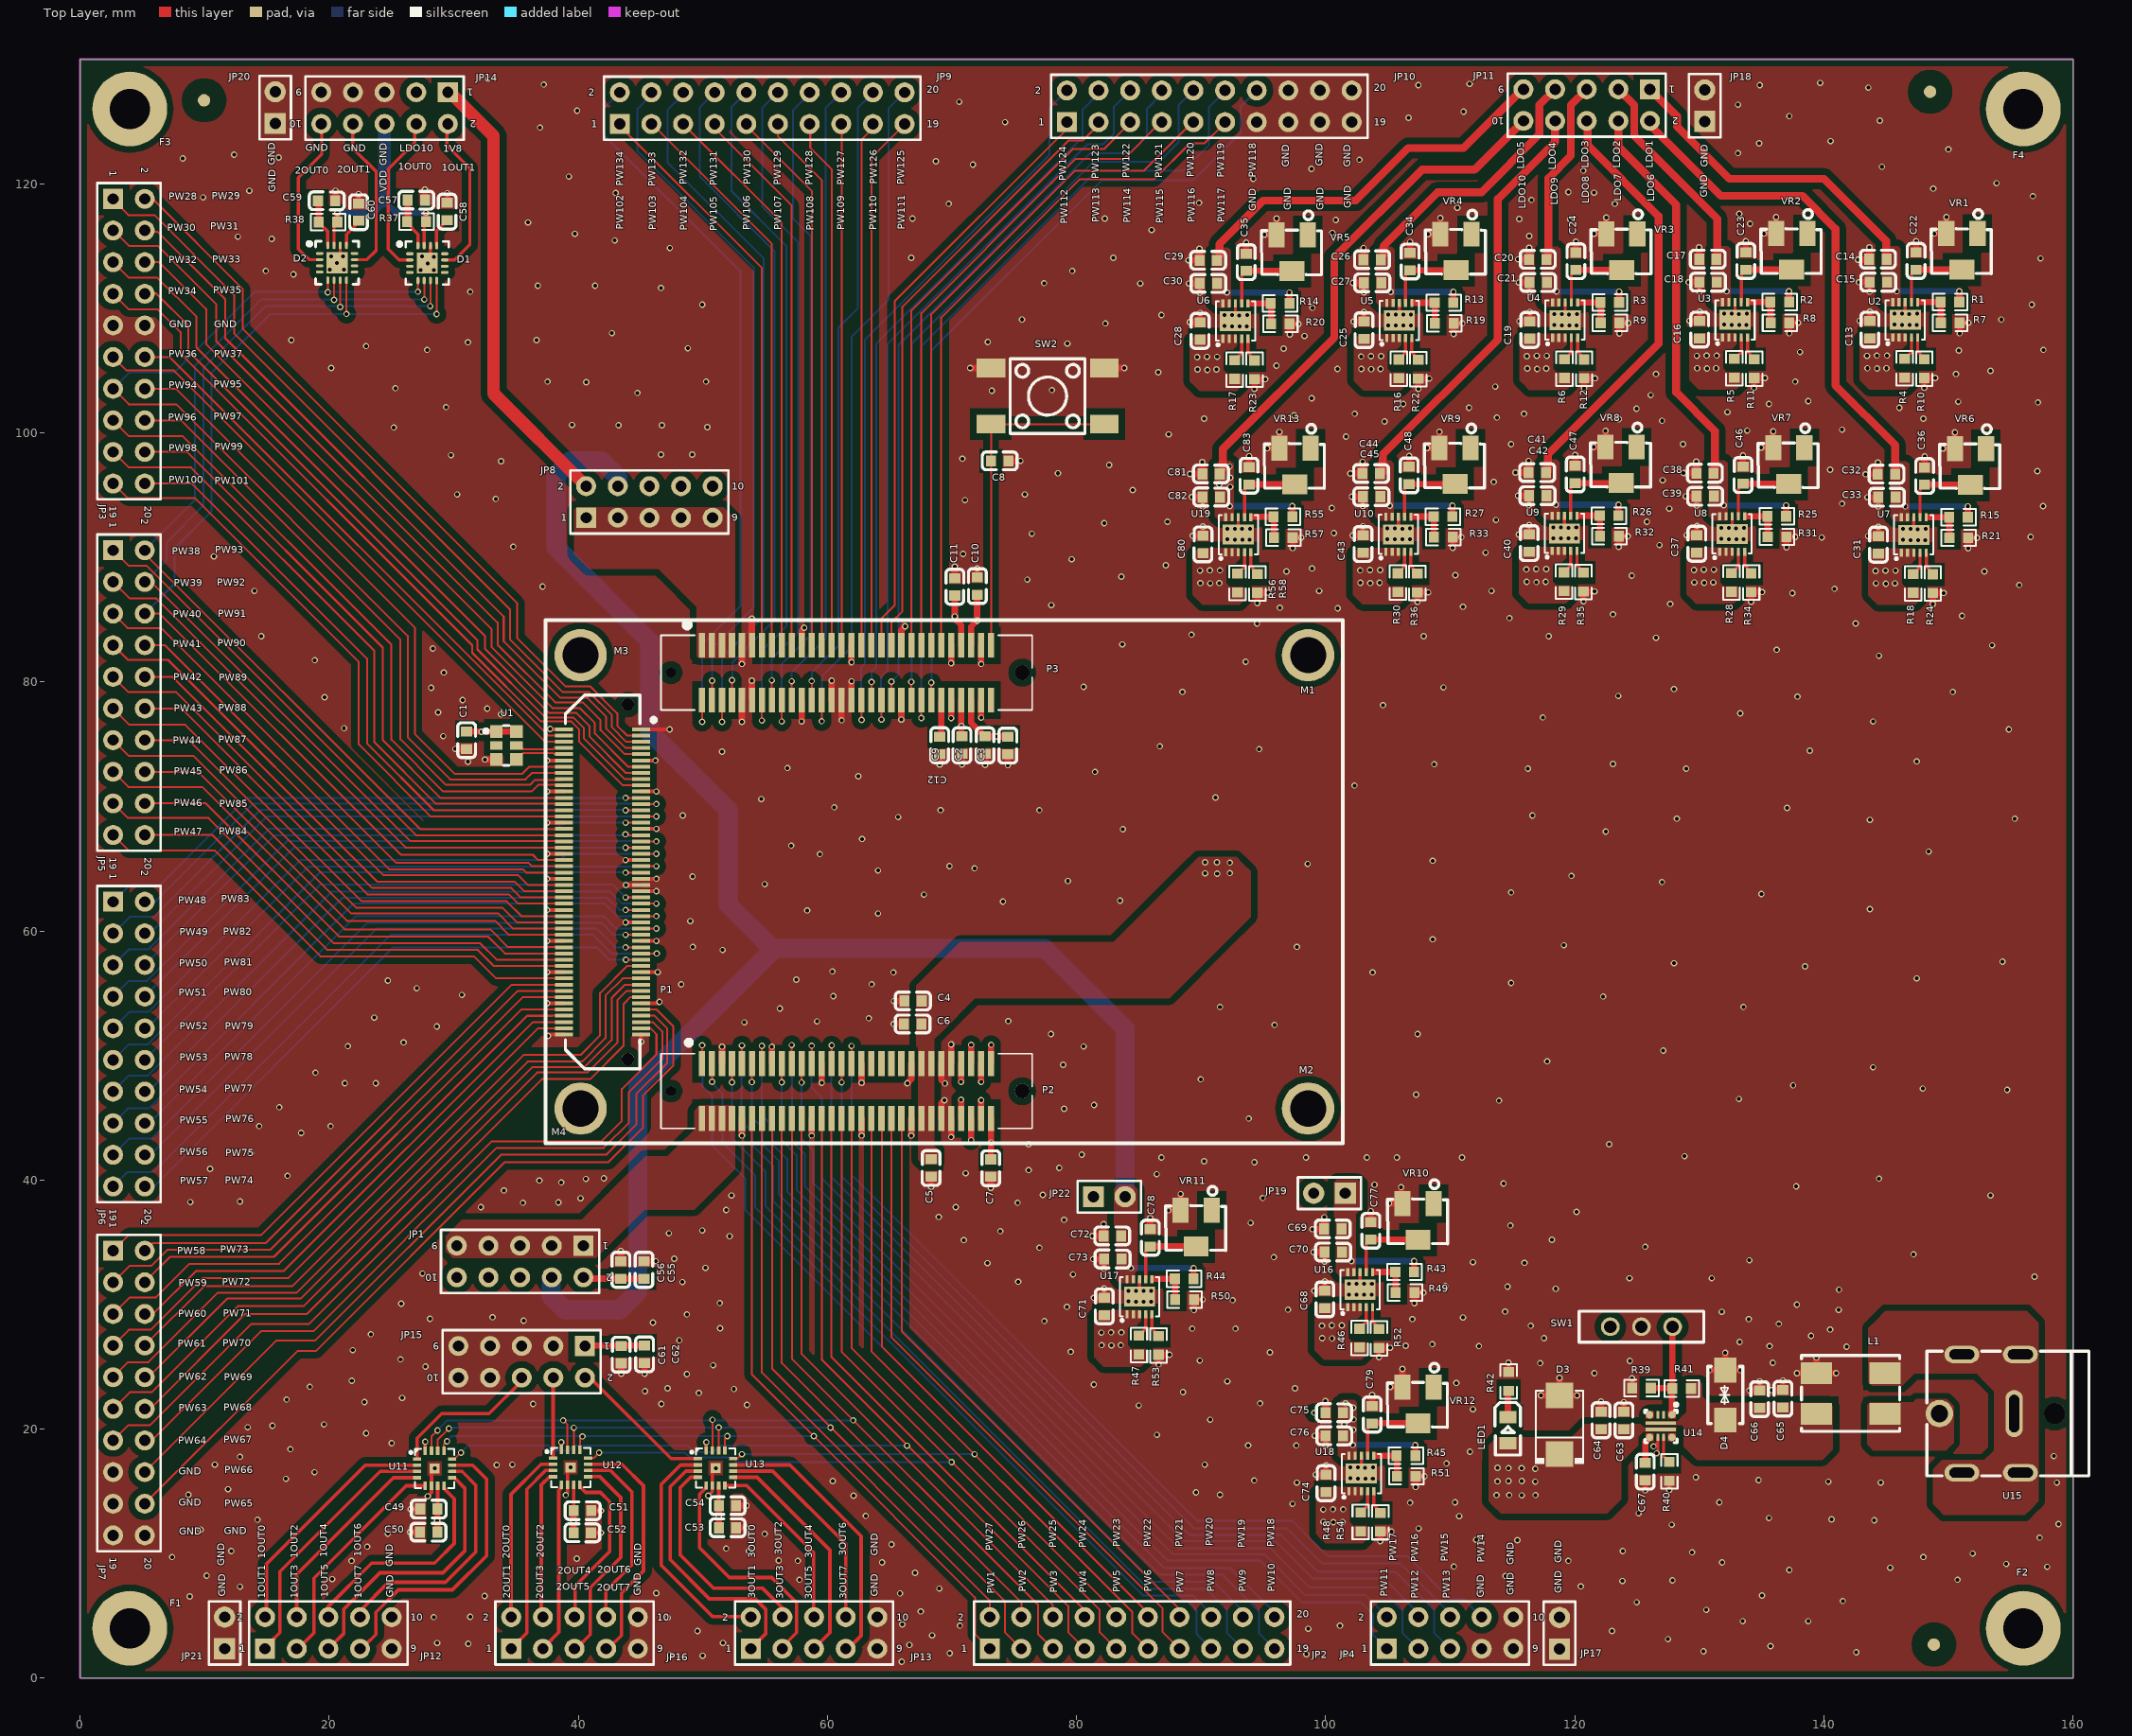
[diagram p0: Top Layer view]
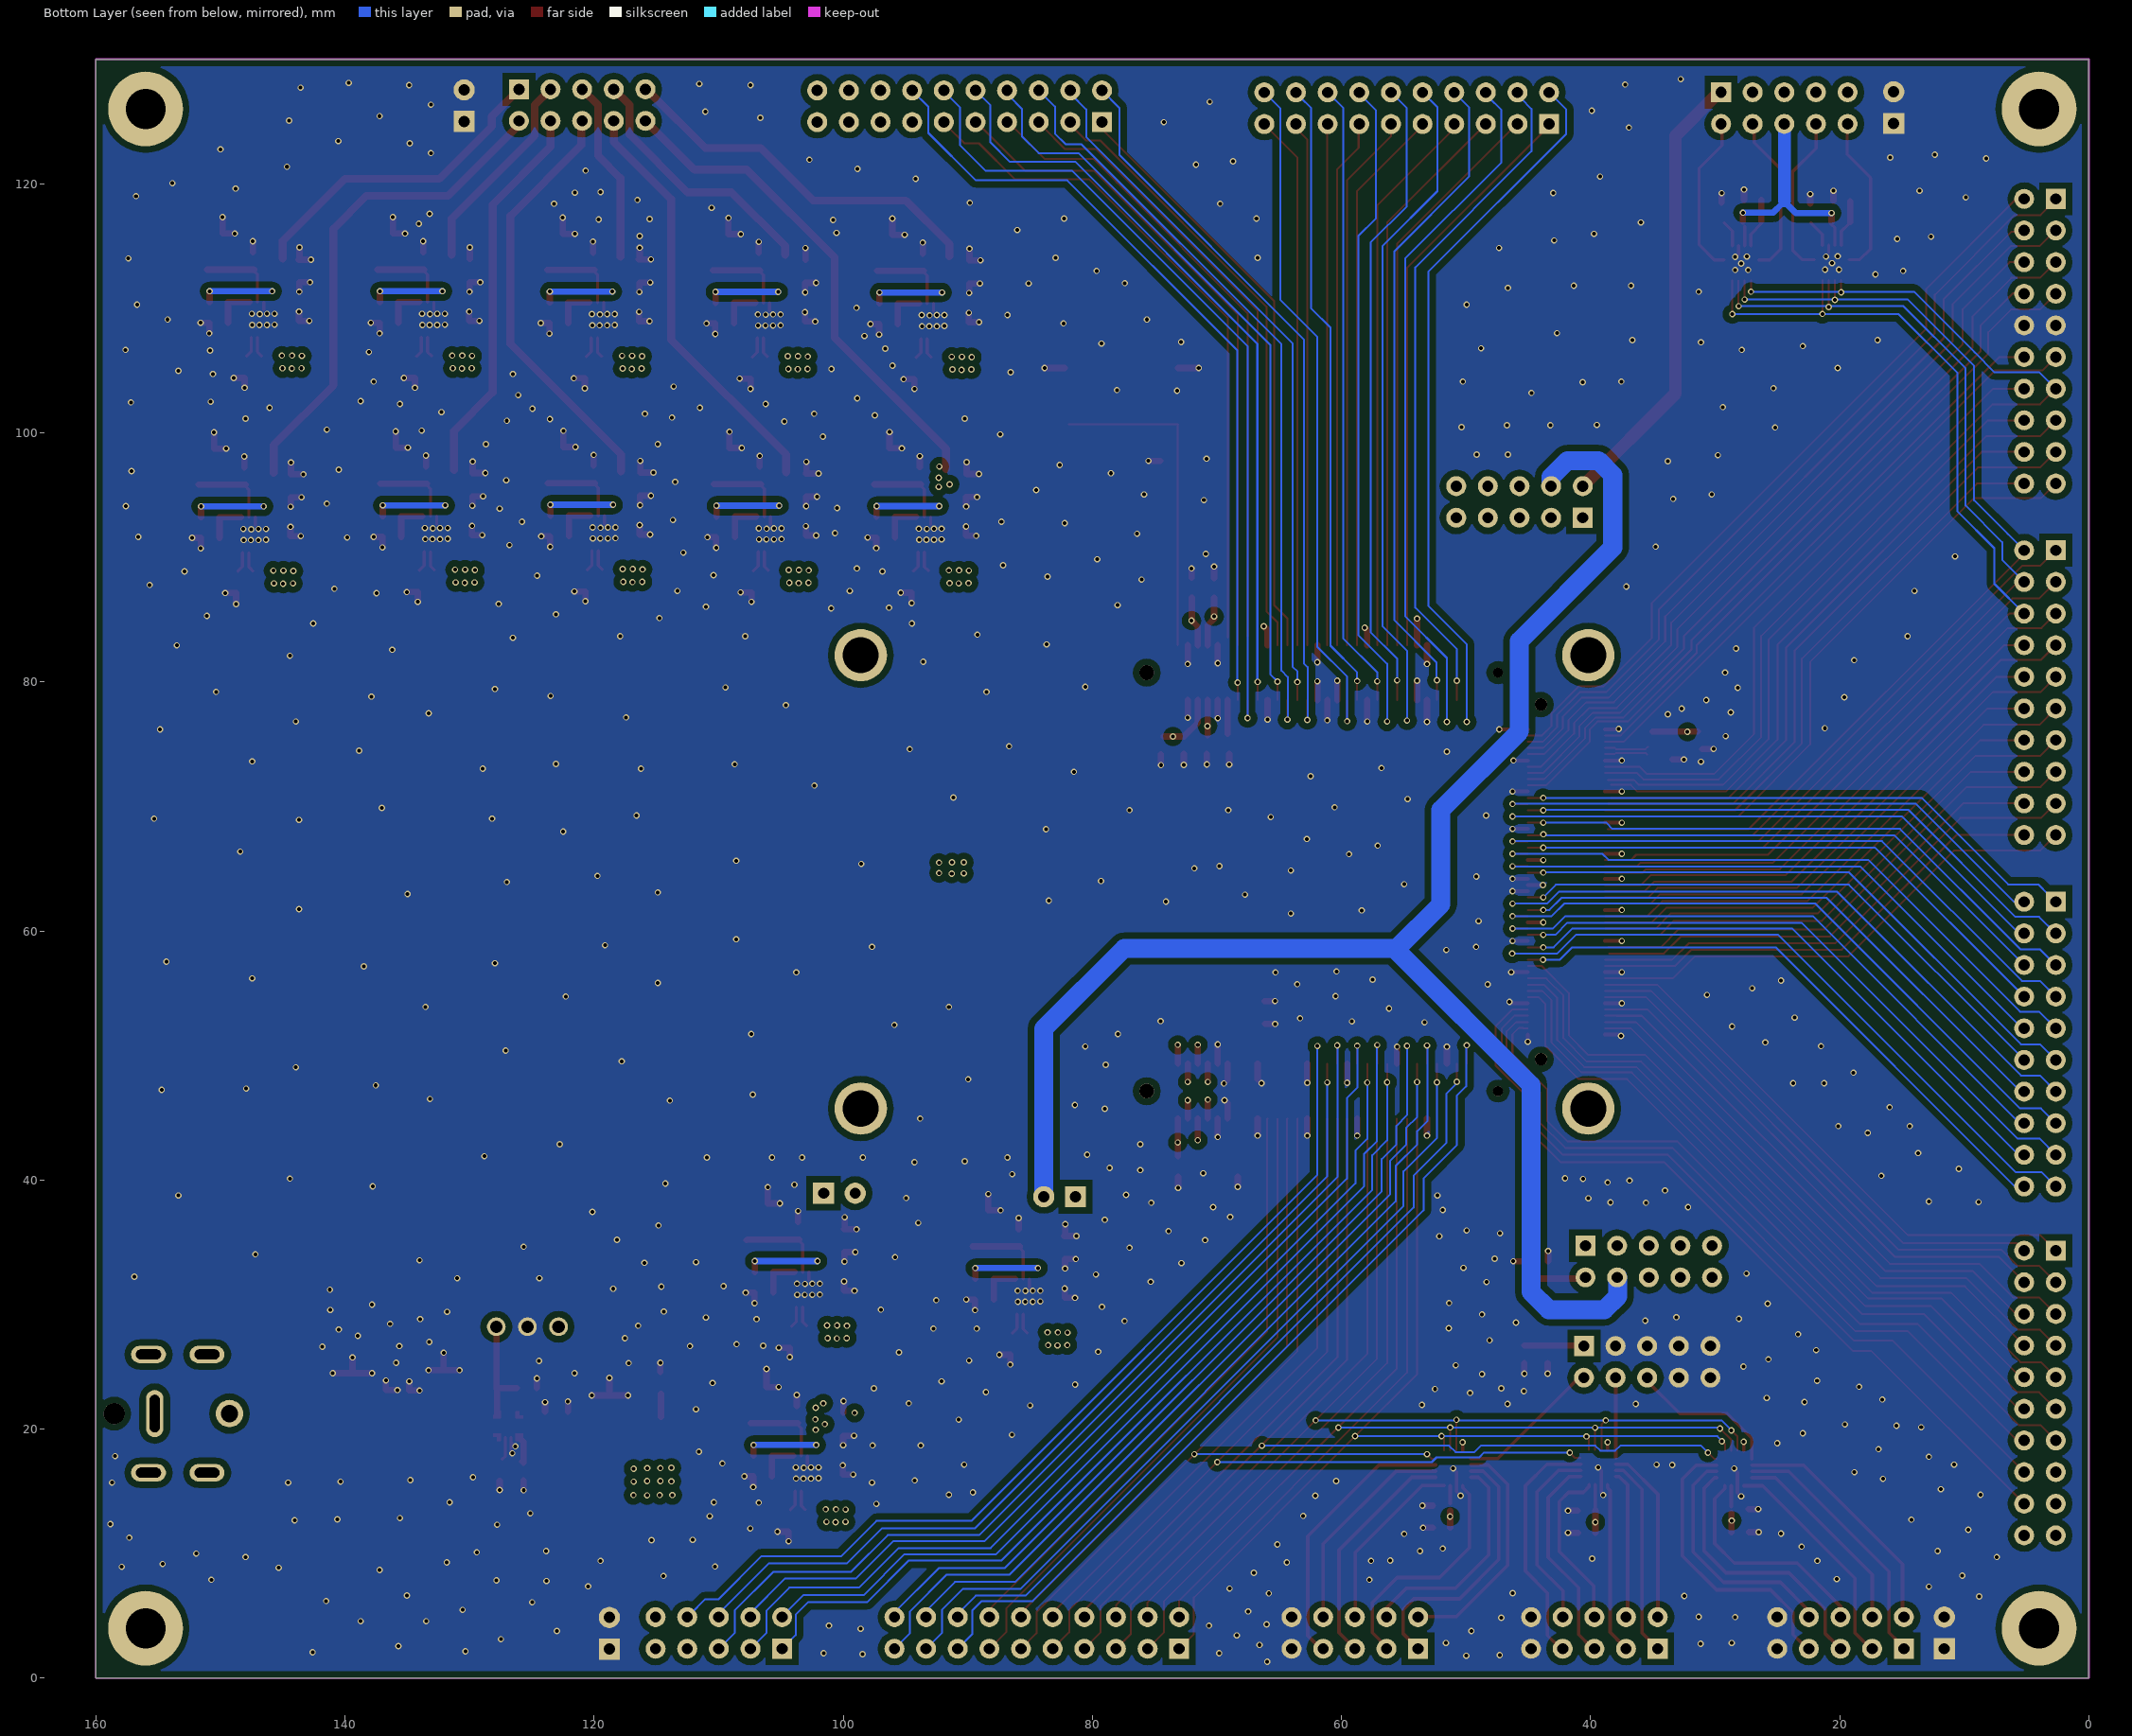
[diagram p1: Bottom Layer view, seen from below]
# Altium PCB MISC82195.PcbDoc (part 1 of 8)
Units mm, origin at the board's own origin, x right, y up, seen from the top; angles counter-clockwise.
Board outline 160 x 130 mm, 4 copper layers (Top Layer, GND, POWER, Bottom Layer); 214 components, 251 nets, 1068 pads, 1218 vias.

## Layer stack, top to bottom (the 12.6 mil dielectric is the usual default, probably not edited)
Top Layer: signal copper 0.0356
Dielectric: core 0.32, FR-4, Dk 4.8
GND: plane copper 0.0356, net GND
Dielectric: prepreg 0.32, FR-4, Dk 4.8
POWER: plane copper 0.0356, net LDO_10
Dielectric: core 0.32, FR-4, Dk 4.8
Bottom Layer: signal copper 0.0356

## Board outline
0,0 160,0 160,130 0,130

## Design rules (kind name [scope] priority, off if disabled: settings)
Clearance Clearance_2 [HASPAD('FREE-MARK')] p1: gap=1.27
Clearance Clearance_1 [INPOLYGON] p2: gap=0.152
Clearance [All] p3: gap=0.152
DiffPairsRouting [All] p1: maxlimit=0.152 minlimit=0.152 mostfreqgap=0.152 maxuncoupledlength=12.7
HoleSize [All] p1: absolutevalues=TRUE maxlimit=12.7 minlimit=0.025 maxpercent=80.000 minpercent=20.000
HoleToHoleClearance [All] p1: gap=0 allowstackedmicrovias=TRUE
MinimumSolderMaskSliver [All] p1: minsoldermaskwidth=0
PlaneClearance [All] p1: clearance=0.152
PlaneConnect [All] p1: planeconnectstyle=Direct reliefexpansion=0.508 reliefentries=4 reliefconductorwidth=0.254 reliefairgap=0.254
PolygonConnect [All] p1: connectstyle=Direct reliefconductorwidth=0.254 reliefentries=4 polygonreliefangle="90 Angle"
RoutingVias [All] p1: holewidth=0.305 width=0.508 viastyle="Through Hole" minholewidth=0.305 minwidth=0.508 maxholewidth=0.305 maxwidth=0.508
SilkToSilkClearance [All] p1: silktosilkclearance=0
SilkscreenOverComponentPads [All] p1: minsilkscreentomaskgap=0
SolderMaskExpansion [All] p1: expansion=0.102
Width [All] p1: maxlimit=2.032 minlimit=0.152 preferedwidth=0.152 minimp=50.000000 maximp=50.000000 favimp=50.000000
20 further rules are at their usual default settings.

## Classes and differential pairs
component class AnalogSignal: C13 C14 C15 C16 C17 C18 C19 C20 C21 C22 C23 C24 C25 C26 C27 C28 C29 C30 C31 C32 C33 C34 C35 C36 C37 C38 C39 C40 C41 C42 C43 C44 C45 C46 C47 C48 C49 C50 C51 C52 C53 C54 C55 C56 C57 C58 C59 C60 C61 C62 C80 C81 C82 C83 C? D1 D2 JP11 JP12 JP13 JP14 JP15 JP16 R1 R2 R3 R4 R5 R6 R7 R8 R9 R10 R11 R12 R13 R14 R15 R16 R17 R18 R19 R20 R21 R22 R23 R24 R25 R26 R27 R28 R29 R30 R31 R32 R33 R34 R35 R36 R37 R38 R55 R56 R57 R58 R? U2 U3 U4 U5 U6 U7 U8 U9 U10 U11 U12 U13 U19 VR1 VR2 VR3 VR4 VR5 VR6 VR7 VR8 VR9 VR13
component class FPGA: C1 C2 C3 C4 C5 C6 C7 C8 C9 C10 C11 C12 F1 F2 F3 F4 JP1 JP2 JP3 JP4 JP5 JP6 JP7 JP8 JP9 JP10 P1 P2 P3 SW2 U1
component class Power: C63 C64 C65 C66 C67 C68 C69 C70 C71 C72 C73 C74 C75 C76 C77 C78 C79 D3 D4 JP17 JP18 JP19 JP20 JP21 JP22 L1 LED1 M1 M2 M3 M4 R39 R40 R41 R42 R43 R44 R45 R46 R47 R48 R49 R50 R51 R52 R53 R54 SW1 U14 U15 U16 U17 U18 VR10 VR11 VR12

## Components (designator, comment, footprint, x,y, rotation, side; value= is the part's Value field where it differs from the comment)
C1 "X7R  100nF/16V" C0603 31.039,75.311 r270 top
C2 "100nF/50V" C0603 72.66,74.915 r90 top
C3 "22uF/10V" C0603 74.489,74.889 r90 top
C4 "100nF/50V" C0603 66.868,54.372 r0 top
C5 "22uF/10V" C0603 68.326,40.97 r90 top
C6 "100nF/50V" C0603 66.853,52.527 r0 top
C7 "100nF/50V" C0603 73.117,40.955 r90 top
C8 "100nF" C0603 73.838,97.739 r0 top
C9 "100nF/50V" C0603 70.806,74.915 r90 top
C10 "100nF/50V" C0603 72.034,87.681 r270 top
C11 "22uF/10V" C0603 70.231,87.63 r270 top
C12 "100nF/50V" C0603 69.012,74.905 r270 top
C13 "10uF" C0603 143.688,108.28 r270 top
C14 "10uF" C0603 144.34,113.944 r0 top
C15 "10uF" C0603 144.366,112.09 r0 top
C16 "10uF" C0603 130.023,108.28 r270 top
C17 "10uF" C0603 130.675,113.944 r0 top
C18 "10uF" C0603 130.701,112.09 r0 top
C19 "10uF" C0603 116.383,108.255 r270 top
C20 "10uF" C0603 117.035,113.919 r0 top
C21 "10uF" C0603 117.061,112.065 r0 top
C22 "4.7uF" C0603 147.388,113.792 r270 top
C23 "4.7uF" C0603 133.723,113.792 r270 top
C24 "4.7uF" C0603 120.083,113.767 r270 top
C25 "10uF" C0603 103.073,108.229 r270 top
C26 "10uF" C0603 103.726,113.894 r0 top
C27 "10uF" C0603 103.751,112.039 r0 top
C28 "10uF" C0603 89.916,108.179 r270 top
C29 "10uF" C0603 90.569,113.843 r0 top
C30 "10uF" C0603 90.594,111.989 r0 top
C31 "10uF" C0603 144.374,91.008 r270 top
C32 "10uF" C0603 145.026,96.672 r0 top
C33 "10uF" C0603 145.052,94.818 r0 top
C34 "4.7uF" C0603 106.774,113.741 r270 top
C35 "4.7uF" C0603 93.617,113.69 r270 top
C36 "4.7uF" C0603 148.074,96.52 r270 top
C37 "10uF" C0603 129.794,91.084 r270 top
C38 "10uF" C0603 130.447,96.749 r0 top
C39 "10uF" C0603 130.472,94.894 r0 top
C40 "10uF" C0603 116.332,91.135 r270 top
C41 "10uF" C0603 116.985,96.799 r0 top
C42 "10uF" C0603 117.01,94.945 r0 top
C43 "10uF" C0603 102.997,91.059 r270 top
C44 "10uF" C0603 103.65,96.723 r0 top
C45 "10uF" C0603 103.675,94.869 r0 top
C46 "4.7uF" C0603 133.495,96.596 r270 top
C47 "4.7uF" C0603 120.033,96.647 r270 top
C48 "4.7uF" C0603 106.698,96.571 r270 top
C49 "10uF" C0603 28.007,13.574 r0 top
C50 "100nF" C0603 27.982,11.72 r0 top
C51 "10uF" C0603 40.344,13.452 r180 top
C52 "100nF" C0603 40.319,11.674 r180 top
C53 "10uF" C0603 51.978,12.08 r180 top
C54 "100nF" C0603 51.978,13.858 r180 top
C55 "0.1uF/16V" C0603 45.272,32.781 r270 top
C56 "0.1uF/16V" C0603 43.418,32.781 r270 top
C57 "100nF" C0603 26.991,118.679 r180 top
C58 "1.5uF" C0603 29.48,117.765 r90 top
C59 "100nF" C0603 19.803,118.628 r180 top
C60 "1.5uF" C0603 22.368,117.714 r90 top
C61 "10uF" C0603 43.443,25.985 r90 top
C62 "10nF" C0603 45.323,26.011 r90 top
C63 "22uF/10V" C0603 123.936,20.691 r270 top
C64 "22uF/10V" C0603 122.098,20.701 r270 top
C65 "X7R 100nF/25V" C0603 136.703,22.428 r270 top
C66 "X7R 100nF/25V" C0603 134.832,22.393 r270 top
C67 "X7R" C0603 125.654,16.586 r90 top
C68 "10uF" C0603 99.924,30.404 r270 top
C69 "10uF" C0603 100.576,36.068 r0 top
C70 "10uF" C0603 100.602,34.214 r0 top
C71 "10uF" C0603 82.22,29.845 r270 top
C72 "10uF" C0603 82.872,35.509 r0 top
C73 "10uF" C0603 82.898,33.655 r0 top
C74 "10uF" C0603 100.025,15.646 r270 top
C75 "10uF" C0603 100.678,21.311 r0 top
C76 "10uF" C0603 100.703,19.456 r0 top
C77 "4.7uF" C0603 103.624,35.916 r270 top
C78 "4.7uF" C0603 85.92,35.357 r270 top
C79 "4.7uF" C0603 103.726,21.158 r270 top
C80 "10uF" C0603 90.145,91.034 r270 top
C81 "10uF" C0603 90.797,96.698 r0 top
C82 "10uF" C0603 90.823,94.844 r0 top
C83 "4.7uF" C0603 93.845,96.545 r270 top
D1 "DAC53202" WQFN-16(3x3) 27.88,113.624 r0 top
D2 "DAC53202" WQFN-16(3x3) 20.641,113.65 r0 top
D3 "#NAME?" SMB_L4.6-W3.6-LS5.3-RD 118.77,20.345 r90 top
D4 "#NAME?" SMA_L4.2-W2.7-LS5.0-BI 132.08,22.733 r270 top
F1 "M3" M3 4,4 r0 top
F2 "M3" M3 156,4 r0 top
F3 "M3" M3 4,126 r0 top
F4 "M3" M3 156,126 r0 top
JP1 "Header 5X2" HDR2.54-LI-2x5P 35.331,33.452 r180 top
JP2 "Header 2X10" HDR2.54-LI-2x10P 84.455,3.632 r0 top
JP3 "Header 2X10" HDR2.54-LI-2x10P 3.928,107.351 r270 top
JP4 "Header 5X2" HDR2.54-LI-2x5P 109.982,3.632 r0 top
JP5 "Header 2X10" HDR2.54-LI-2x10P 3.928,79.131 r270 top
JP6 "Header 2X10" HDR2.54-LI-2x10P 3.928,50.912 r270 top
JP7 "Header 2X10" HDR2.54-LI-2x10P 3.928,22.896 r270 top
JP8 "Header 5X2" HDR2.54-LI-2x5P 45.711,94.447 r0 top
JP9 "Header 2X10" HDR2.54-LI-2x10P 54.762,126.06 r0 top
JP10 "Header 2X10" HDR2.54-LI-2x10P 90.653,126.213 r0 top
JP11 "Header 5X2" HDR2.54-LI-2x5P 120.955,126.314 r180 top
JP12 "Header 5X2" HDR2.54-LI-2x5P 19.939,3.632 r0 top
JP13 "Header 5X2" HDR2.54-LI-2x5P 58.928,3.632 r0 top
JP14 "Header 5X2" HDR2.54-LI-2x5P 24.451,126.07 r180 top
JP15 "Header 5X2" HDR2.54-LI-2x5P 35.458,25.4 r180 top
JP16 "Header 5X2" HDR2.54-LI-2x5P 39.7,3.632 r0 top
JP17 "HDR-1X2" HDR2.54-LI-2P 118.77,3.607 r90 top
JP18 "HDR-1X2" HDR2.54-LI-2P 130.429,126.263 r90 top
JP19 "HDR-1X2" HDR2.54-LI-2P 100.305,38.938 r180 top
JP20 "HDR-1X2" HDR2.54-LI-2P 15.672,126.111 r90 top
JP21 "HDR-1X2" HDR2.54-LI-2P 11.608,3.632 r90 top
JP22 "HDR-1X2" HDR2.54-LI-2P 82.626,38.659 r0 top
L1 "#NAME?" FILTER-SMD_4P-L7.0-W6.0-TL_SMCM7060 142.138,22.86 r180 top
LED1 "#NAME?" LED0805-R-RD 114.63,19.914 r270 top
M1 "M2-4-L5-1.6" M2.9 83.167,80.738 r0 top
M2 "M2-4-L5-1.6" M2.9 83.167,44.338 r0 top
M3 "M2-4-L5-1.6" M2.9 24.767,80.738 r0 top
M4 "M2-4-L5-1.6" M2.9 24.767,44.338 r0 top
P1 "XMS6302-B" XMS6302-B 41.952,63.938 r270 top locked
P2 "XMS6302-A" XMS6302-A 61.537,47.138 r0 top locked
P3 "XMS6302-C" XMS6302-C 61.537,80.739 r0 top locked
R1 "453k" R0603 150.106,110.49 r0 top
R2 "453k" R0603 136.441,110.49 r0 top
R3 "453k" R0603 122.801,110.465 r0 top
R4 "200k" R0603 146.474,105.181 r270 top
R5 "200k" R0603 132.809,105.181 r270 top
R6 "200k" R0603 119.169,105.156 r270 top
R7 "50k" R0603 150.132,108.839 r180 top
R8 "50k" R0603 136.466,108.839 r180 top
R9 "50k" R0603 122.827,108.814 r180 top
R10 "249R" R0603 148.049,105.156 r90 top
R11 "249R" R0603 134.384,105.156 r90 top
R12 "249R" R0603 120.744,105.131 r90 top
R13 "453k" R0603 109.492,110.439 r0 top
R14 "453k" R0603 96.334,110.388 r0 top
R15 "453k" R0603 150.792,93.218 r0 top
R16 "200k" R0603 105.859,105.131 r270 top
R17 "200k" R0603 92.702,105.08 r270 top
R18 "200k" R0603 147.16,87.909 r270 top
R19 "50k" R0603 109.517,108.788 r180 top
R20 "50k" R0603 96.36,108.737 r180 top
R21 "50k" R0603 150.817,91.567 r180 top
R22 "249R" R0603 107.434,105.105 r90 top
R23 "249R" R0603 94.277,105.054 r90 top
R24 "249R" R0603 148.735,87.884 r90 top
R25 "453k" R0603 136.212,93.294 r0 top
R26 "453k" R0603 122.75,93.345 r0 top
R27 "453k" R0603 109.415,93.269 r0 top
R28 "200k" R0603 132.58,87.986 r270 top
R29 "200k" R0603 119.118,88.036 r270 top
R30 "200k" R0603 105.783,87.96 r270 top
R31 "50k" R0603 136.238,91.643 r180 top
R32 "50k" R0603 122.776,91.694 r180 top
R33 "50k" R0603 109.441,91.618 r180 top
R34 "249R" R0603 134.155,87.96 r90 top
R35 "249R" R0603 120.693,88.011 r90 top
R36 "249R" R0603 107.358,87.935 r90 top
R37 "10K" R0603 27.016,116.952 r0 top
R38 "10K" R0603 19.904,116.926 r0 top
R39 "357K" R0603 125.349,23.292 r180 top
R40 "681Ω" R0603 127.584,16.612 r270 top
R41 "1M" R0603 128.575,23.266 r180 top
R42 "10K" R0603 114.681,23.825 r270 top
R43 "453k" R0603 106.342,32.614 r0 top
R44 "453k" R0603 88.638,32.055 r0 top
R45 "453k" R0603 106.444,17.856 r0 top
R46 "200k" R0603 102.71,27.305 r270 top
R47 "200k" R0603 85.006,26.746 r270 top
R48 "200k" R0603 102.811,12.548 r270 top
R49 "50k" R0603 106.367,30.963 r180 top
R50 "50k" R0603 88.664,30.404 r180 top
R51 "50k" R0603 106.469,16.205 r180 top
R52 "249R" R0603 104.285,27.28 r90 top
R53 "249R" R0603 86.581,26.721 r90 top
R54 "249R" R0603 104.386,12.522 r90 top
R55 "453k" R0603 96.563,93.243 r0 top
R56 "200k" R0603 92.931,87.935 r270 top
R57 "50k" R0603 96.588,91.592 r180 top
R58 "249R" R0603 94.506,87.909 r90 top
SW1 "#NAME?" SW-TH_K3-1204D 125.349,28.219 r0 top
SW2 "Key_SMD_6x6x6.5" SW-SMD_4P-L6.0-W6.0-P4.50-LS9.0-2 77.673,102.946 r0 top
U1 "SiT9121AI-2B1-XXE100" 3225-6p 34.23,74.889 r270 top
U2 "#NAME?" DFN-10_L3.0-W3.0-P0.50-BL-EP-3 146.525,109.068 r0 top
U3 "#NAME?" DFN-10_L3.0-W3.0-P0.50-BL-EP-3 132.86,109.068 r0 top
U4 "#NAME?" DFN-10_L3.0-W3.0-P0.50-BL-EP-3 119.22,109.042 r0 top
U5 "#NAME?" DFN-10_L3.0-W3.0-P0.50-BL-EP-3 105.91,109.017 r0 top
U6 "#NAME?" DFN-10_L3.0-W3.0-P0.50-BL-EP-3 92.753,108.966 r0 top
U7 "#NAME?" DFN-10_L3.0-W3.0-P0.50-BL-EP-3 147.211,91.796 r0 top
U8 "#NAME?" DFN-10_L3.0-W3.0-P0.50-BL-EP-3 132.631,91.872 r0 top
U9 "#NAME?" DFN-10_L3.0-W3.0-P0.50-BL-EP-3 119.169,91.923 r0 top
U10 "#NAME?" DFN-10_L3.0-W3.0-P0.50-BL-EP-3 105.834,91.846 r0 top
U11 "DAC60508ZRTER" WQFN-16_L3.0-W3.0-P0.50-BL-EP0.8 28.464,16.85 r270 top
U12 "DAC60508ZRTER" WQFN-16_L3.0-W3.0-P0.50-BL-EP0.8 39.386,16.927 r270 top
U13 "DAC60508ZRTER" WQFN-16_L3.0-W3.0-P0.50-BL-EP0.8 51.019,16.876 r270 top
U14 "#NAME?" VQFN-10_L2.0-W2.0-P0.45-TL 126.898,20.244 r270 top
U15 "#NAME?" DC-IN-TH_HX-DC007B-2.5 152.518,21.245 r180 top
U16 "#NAME?" DFN-10_L3.0-W3.0-P0.50-BL-EP-3 102.761,31.191 r0 top
U17 "#NAME?" DFN-10_L3.0-W3.0-P0.50-BL-EP-3 85.057,30.632 r0 top
U18 "#NAME?" DFN-10_L3.0-W3.0-P0.50-BL-EP-3 102.862,16.434 r0 top
U19 "#NAME?" DFN-10_L3.0-W3.0-P0.50-BL-EP-3 92.982,91.821 r0 top
VR1 "50kΩ" RES-ADJ-SMD_3224W 151.071,114.554 r180 top
VR2 "50kΩ" RES-ADJ-SMD_3224W 137.406,114.554 r180 top
VR3 "50kΩ" RES-ADJ-SMD_3224W 123.766,114.529 r180 top
VR4 "50kΩ" RES-ADJ-SMD_3224W 110.457,114.503 r180 top
VR5 "50kΩ" RES-ADJ-SMD_3224W 97.3,114.452 r180 top
VR6 "50kΩ" RES-ADJ-SMD_3224W 151.757,97.282 r180 top
VR7 "50kΩ" RES-ADJ-SMD_3224W 137.178,97.358 r180 top
VR8 "50kΩ" RES-ADJ-SMD_3224W 123.716,97.409 r180 top